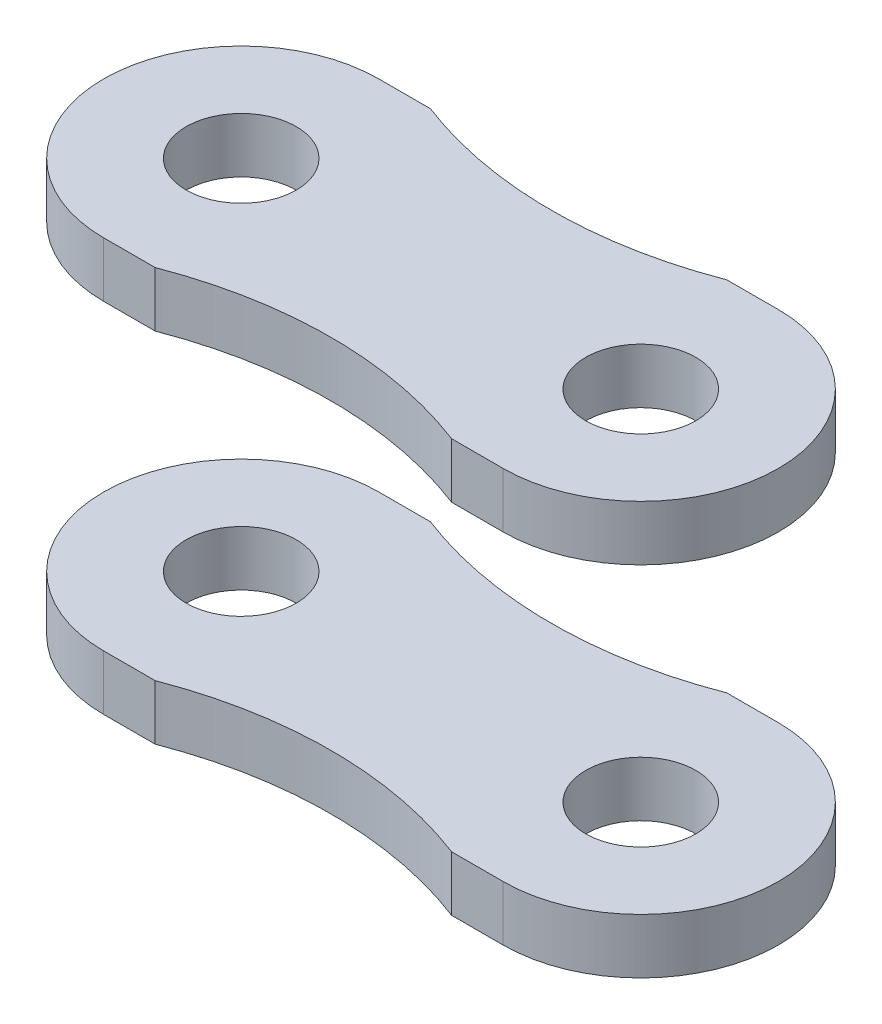
SolidWorks part; units mm, degrees
ref_plane "Front Plane" through (0, 0, 0) normal (0, 0, 1) x (1, 0, 0)
ref_plane "Top Plane" through (0, 0, 0) normal (0, 1, 0) x (1, 0, 0)
ref_plane "Right Plane" through (0, 0, 0) normal (1, 0, 0) x (0, 0, -1)
other "Configuration Table"
sketch "Sketch1" plane through (0, 0, 0) normal (0, 1, 0) x (1, 0, 0)
  line L0 (0, 0) -> (14.52, 0) construction
  line L1 (0, 5) -> (14.52, 5)
  line L2 (0, -5) -> (14.52, -5)
  arc A0 (0, 5) -> (0, -5) centre (0, 0) ccw
  arc A1 (14.52, -5) -> (14.52, 5) centre (14.52, 0) ccw
  circle A2 centre (0, 0) radius 2
  circle A3 centre (14.52, 0) radius 2
  point P3 (7.26, 0)
  dimension "D2" = 5
  dimension "D1" = 14.52
extrude "Boss-Extrude1" add sketch "Sketch1" along normal blind 15
ref_plane "Plane2" through (0, 7.5, 0) normal (0, 1, 0) x (1, 0, 0)
sketch "Sketch2" plane through (0, 7.5, 0) normal (0, 1, 0) x (1, 0, 0)
  line L0 (0, 0) -> (14.52, 0) construction
  line L1 (0, 6.9017) -> (14.52, 6.9017)
  line L2 (0, -6.9017) -> (14.52, -6.9017)
  arc A0 (0, 6.9017) -> (0, -6.9017) centre (0, 0) ccw
  arc A1 (14.52, -6.9017) -> (14.52, 6.9017) centre (14.52, 0) ccw
  point P4 (7.26, 0)
extrude "Cut-Extrude1" cut sketch "Sketch2" against normal blind 5.5 and the other way blind 5.5
sketch "Sketch3" plane through (0, 7.5, 0) normal (0, 1, 0) x (1, 0, 0)
  point P0 (0, 0)
  point P1 (14.52, 0)
sketch "Sketch4" plane through (0, 15, 0) normal (0, 1, 0) x (1, 0, 0)
  line L0 (0, 0) -> (14.52, 0) construction
  line L1 (7.26, 17) -> (7.26, -17) construction
  line L3 (14.52, 5) -> (0, 5) construction
  line L4 (0, -5) -> (14.52, -5) construction
  circle A0 centre (7.26, 19) radius 15
  circle A1 centre (7.26, -19) radius 15
  point P7 (7.26, 0)
  dimension "D1" = 30
  dimension "D2" = 30
  dimension "D3" = 14
  dimension "D4" = 14
extrude "Cut-Extrude2" cut sketch "Sketch4" against normal blind 15
